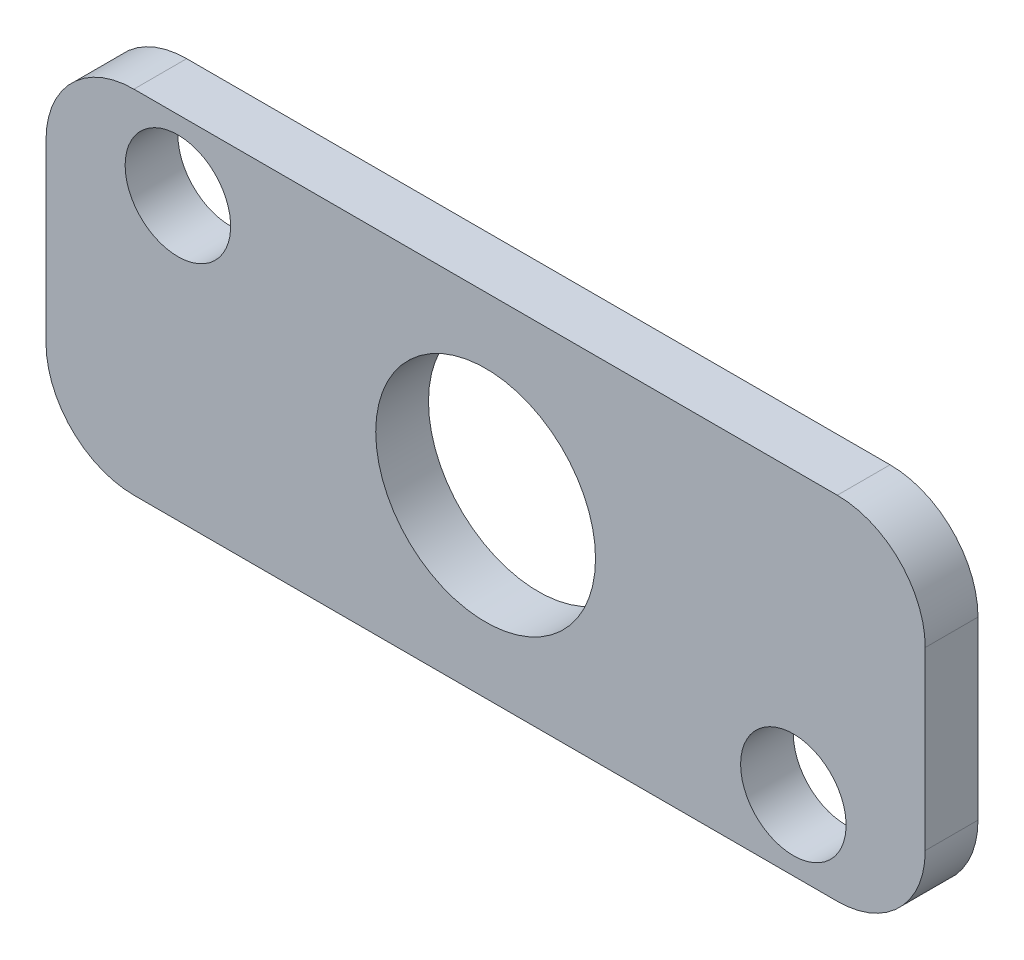
from build123d import *

# Parameters (mm, degrees)
SKETCH_1_R      = 3
SKETCH_1_R_2    = 6.25
EXTRUDE_1_DEPTH = 3


with BuildPart() as part:
    # 草图1 → 凸台-拉伸1 (new body)
    with BuildSketch(Plane.XY.offset(1.5)):
        with BuildLine():
            Line((-20, -10), (20, -10))
            ThreePointArc((20, -10), (23.535533906, -8.535533906), (25, -5))
            Line((25, -5), (25, 5))
            ThreePointArc((25, 5), (23.535533906, 8.535533906), (20, 10))
            Line((20, 10), (-20, 10))
            ThreePointArc((-20, 10), (-23.535533906, 8.535533906), (-25, 5))
            Line((-25, 5), (-25, -5))
            ThreePointArc((-25, -5), (-23.535533906, -8.535533906), (-20, -10))
        make_face()
        with Locations(Location((-17.5, 6, 0), (0, 0, 180))):
            Circle(SKETCH_1_R, mode=Mode.SUBTRACT)
        with Locations(Location((17.5, -6, 0), (0, 0, 180))):
            Circle(SKETCH_1_R, mode=Mode.SUBTRACT)
        with Locations(Location((0, 0, 0), (0, 0, 180))):
            Circle(SKETCH_1_R_2, mode=Mode.SUBTRACT)
    extrude(amount=-EXTRUDE_1_DEPTH)


solid = part.part
